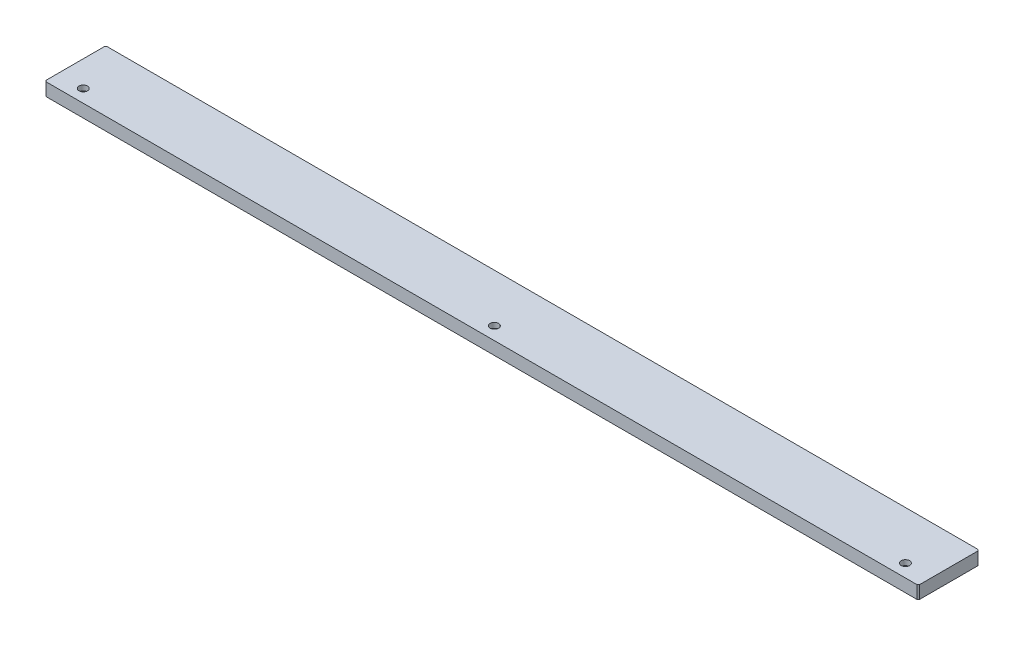
from build123d import *

# Parameters (mm, degrees)
SKETCH_1_W                  = 680
SKETCH_1_H                  = 47.5
EXTRUDE_1_DEPTH             = 5
CHAMFER_1_SIZE              = 1
HOLE_WIZARD_1_D             = 6.6
HOLE_WIZARD_1_CBORE_D       = 11
HOLE_WIZARD_1_CBORE_DEPTH   = 6
HOLE_WIZARD_4_1_4_1_1_D     = 4.1
HOLE_WIZARD_4_1_4_1_1_DEPTH = 10
HOLE_WIZARD_4_1_4_1_1_TIP   = 1.231764269


with BuildPart() as part:
    # 草图1 → 凸台-拉伸1 (new, symmetric)
    with BuildSketch(Plane(origin=(0, 0, 0), x_dir=(1, 0, 0), z_dir=(0, 1, 0))):
        Rectangle(SKETCH_1_W, SKETCH_1_H)
    extrude(amount=EXTRUDE_1_DEPTH, both=True)

    # 倒角1
    chamfer_1_edges = [part.edges().sort_by_distance(p)[0] for p in [
        (340, 0, 23.75),
        (-340, 0, 23.75),
        (-340, 0, -23.75),
        (340, 0, -23.75),
    ]]
    chamfer(chamfer_1_edges, length=CHAMFER_1_SIZE)

    # 打孔尺寸(%根据)内六角圆柱头螺钉的类型1 (through all)
    with Locations(Plane(origin=(0, -5, 0), x_dir=(-1, 0, 0), z_dir=(0, -1, 0))):
        with Locations((-320, -13.75), (0, -13.75), (320, -13.75)):
            CounterBoreHole(HOLE_WIZARD_1_D / 2, HOLE_WIZARD_1_CBORE_D / 2, HOLE_WIZARD_1_CBORE_DEPTH)

    # Ø4.1 (4.1) 直径孔1
    with Locations(Plane(origin=(0, 0, -23.75), x_dir=(-1, 0, 0), z_dir=(0, 0, -1))):
        with Locations((-320, 0), (-300, 0), (-280, 0), (-260, 0), (-240, 0), (-220, 0), (-200, 0), (-180, 0), (-160, 0), (-140, 0), (-120, 0), (-100, 0), (-80, 0), (-60, 0), (-40, 0), (-20, 0), (0, 0), (20, 0), (40, 0), (60, 0), (80, 0), (100, 0), (120, 0), (140, 0), (160, 0), (180, 0), (200, 0), (220, 0), (240, 0), (260, 0), (280, 0), (300, 0), (320, 0)):
            Hole(HOLE_WIZARD_4_1_4_1_1_D / 2, depth=HOLE_WIZARD_4_1_4_1_1_DEPTH)
            with Locations((0, 0, -(HOLE_WIZARD_4_1_4_1_1_DEPTH + HOLE_WIZARD_4_1_4_1_1_TIP / 2))):  # 118° drill point
                Cone(0, HOLE_WIZARD_4_1_4_1_1_D / 2, HOLE_WIZARD_4_1_4_1_1_TIP, mode=Mode.SUBTRACT)


solid = part.part
